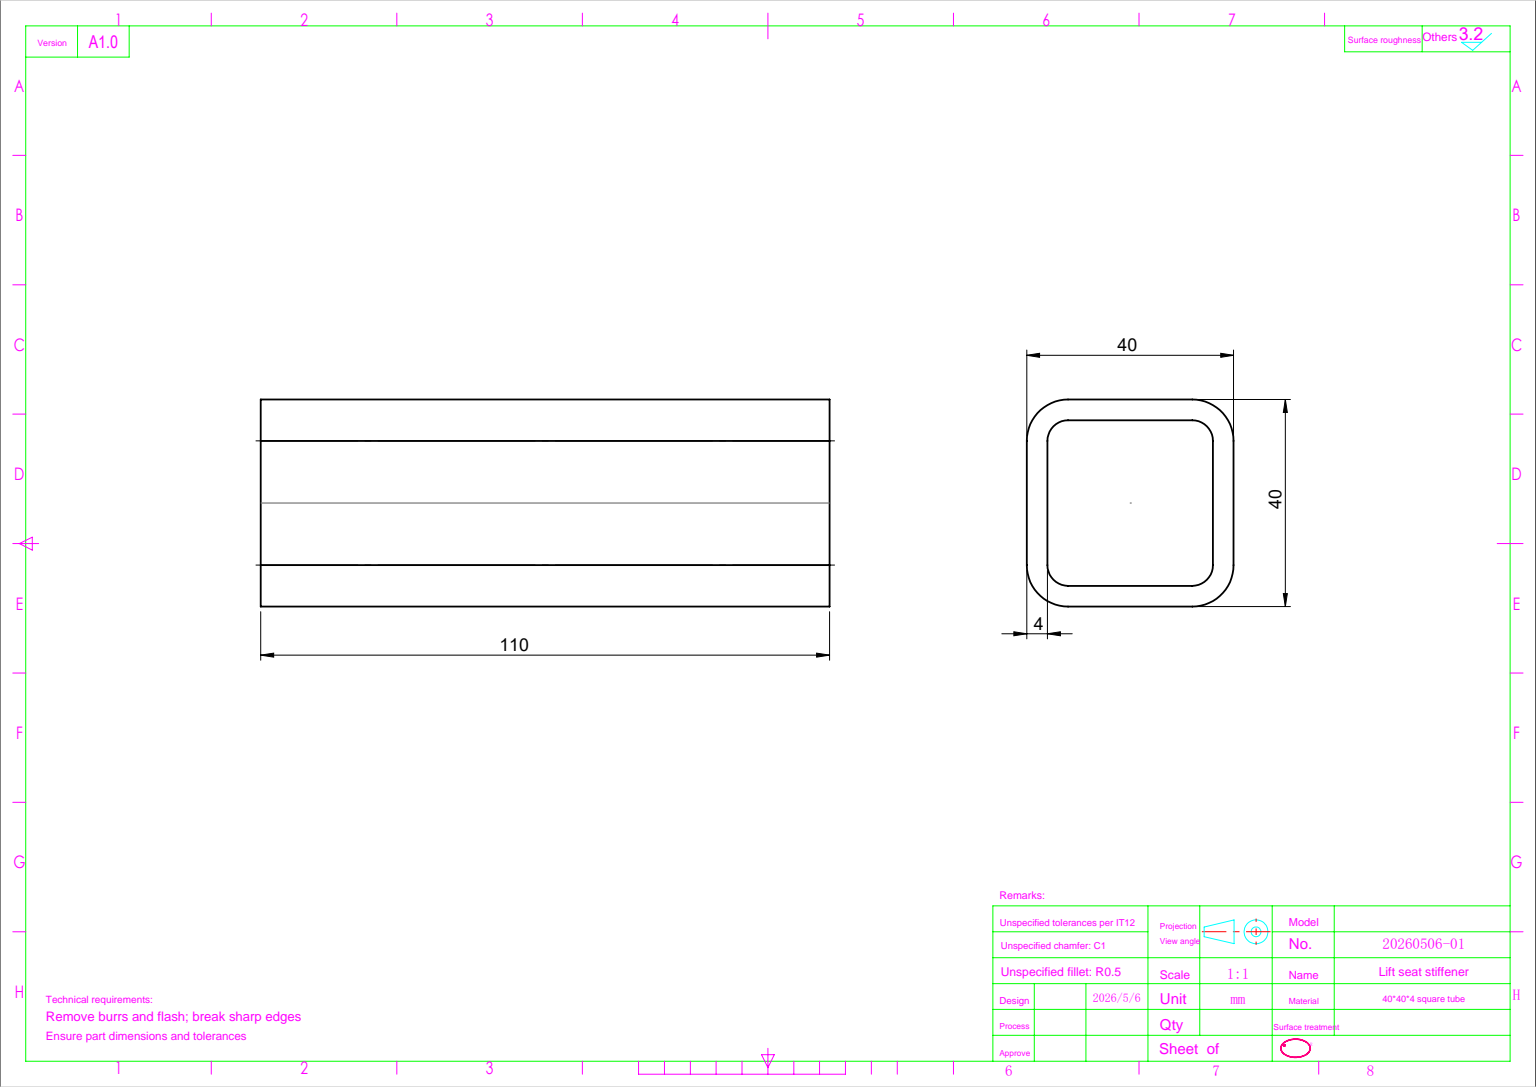
SolidWorks part; units mm, degrees
ref_plane "前视基准面" through (0, 0, 0) normal (0, 0, 1) x (1, 0, 0)
ref_plane "上视基准面" through (0, 0, 0) normal (0, 1, 0) x (1, 0, 0)
ref_plane "右视基准面" through (0, 0, 0) normal (1, 0, 0) x (0, 0, -1)
sketch3d "3D草图1"
  line L0 (0, 0, 0) -> (110, 0, 0)
  dimension "D1" = 110
other "方形管 40 X 40 X 4(1)"
ref_plane "基准面1" through (0, 0, 0) normal (1, 0, 0) x (0, 0, -1)
sketch "Sketch12" plane through (0, 0, 0) normal (1, 0, 0) x (0, 0, -1)
  line L0 (-12, -16) -> (12, -16)
  line L1 (-16, -12) -> (-16, 12)
  line L2 (12, 16) -> (-12, 16)
  line L3 (16, 12) -> (16, -12)
  line L4 (-12, -20) -> (12, -20)
  line L5 (-20, -12) -> (-20, 12)
  line L6 (12, 20) -> (-12, 20)
  line L7 (20, 12) -> (20, -12)
  arc A0 (20, 12) -> (12, 20) centre (12, 12) ccw
  arc A1 (12, -20) -> (20, -12) centre (12, -12) ccw
  arc A2 (-20, -12) -> (-12, -20) centre (-12, -12) ccw
  arc A3 (-12, 20) -> (-20, 12) centre (-12, 12) ccw
  arc A4 (-12, 16) -> (-16, 12) centre (-12, 12) ccw
  arc A5 (16, 12) -> (12, 16) centre (12, 12) ccw
  arc A6 (12, -16) -> (16, -12) centre (12, -12) ccw
  arc A7 (-16, -12) -> (-12, -16) centre (-12, -12) ccw
  point P0 (-20, 0)
  point P1 (20, 0)
  point P2 (0, 20)
  point P3 (0, -20)
  point P4 (0, 0)
  point P5 (-20, -20)
  point P6 (20, -20)
  point P7 (20, 20)
  point P8 (-20, 20)
  point P33 (0, 0)
  dimension "D1" = 8
  dimension "Thickness" = 4
  dimension "V_leg" = 40
